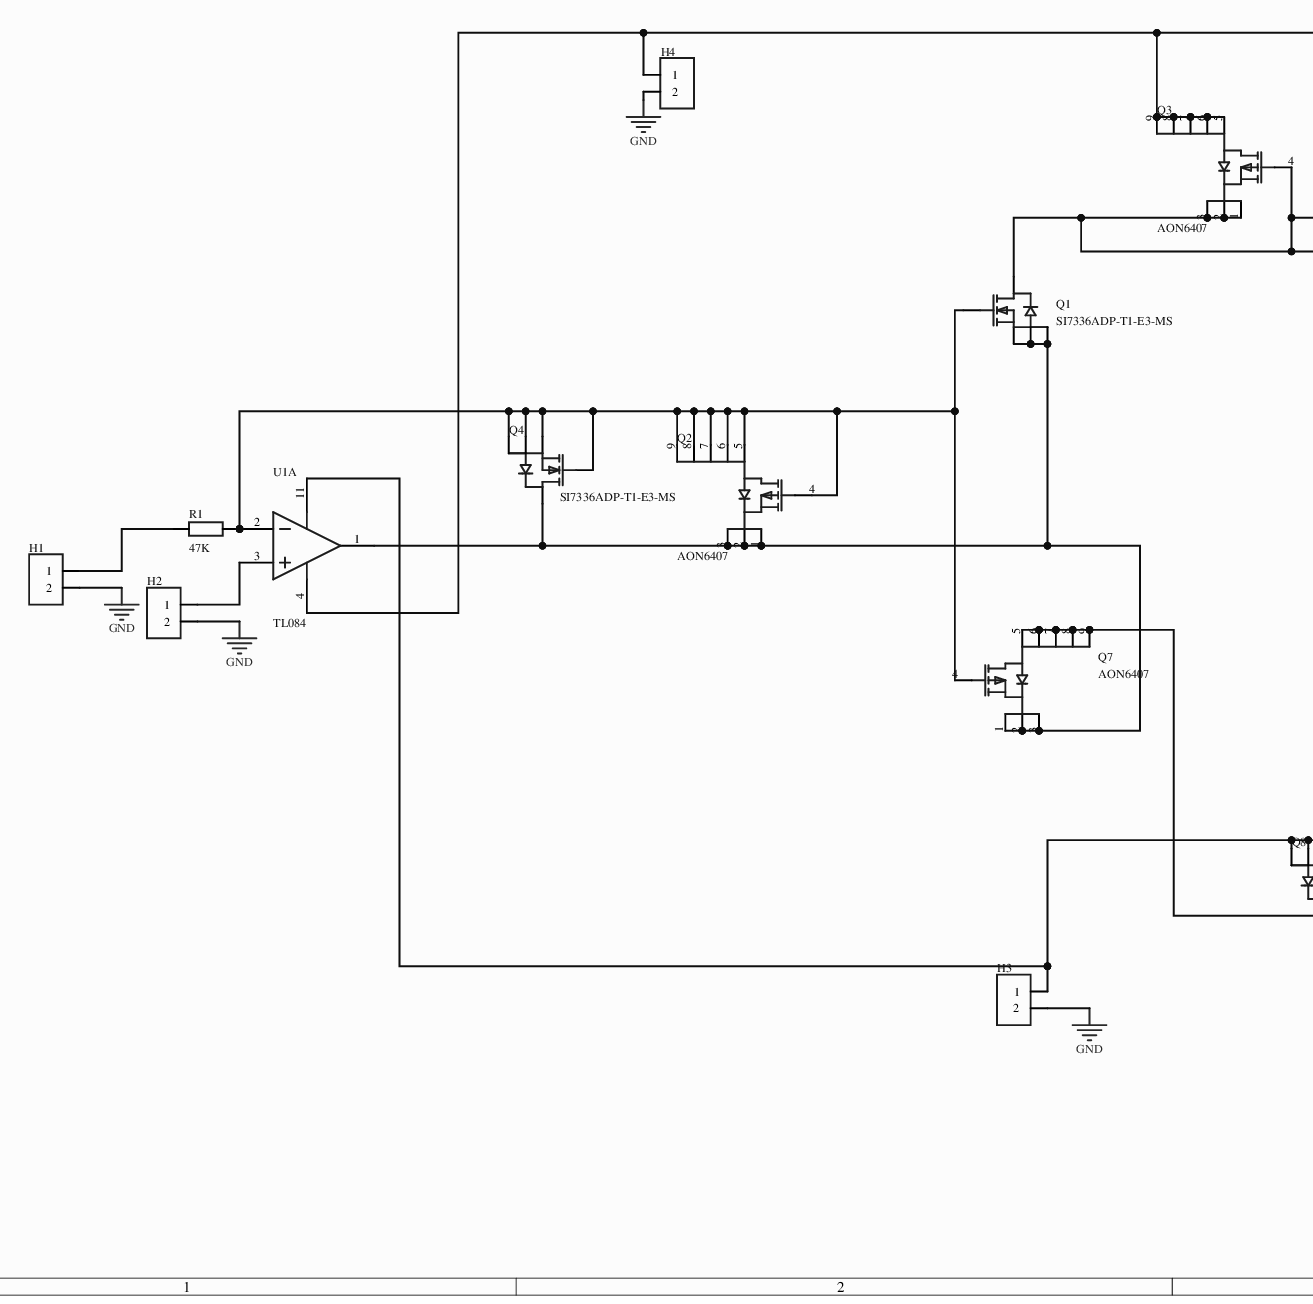
[diagram p0: MISC51994-3.schdoc, left]
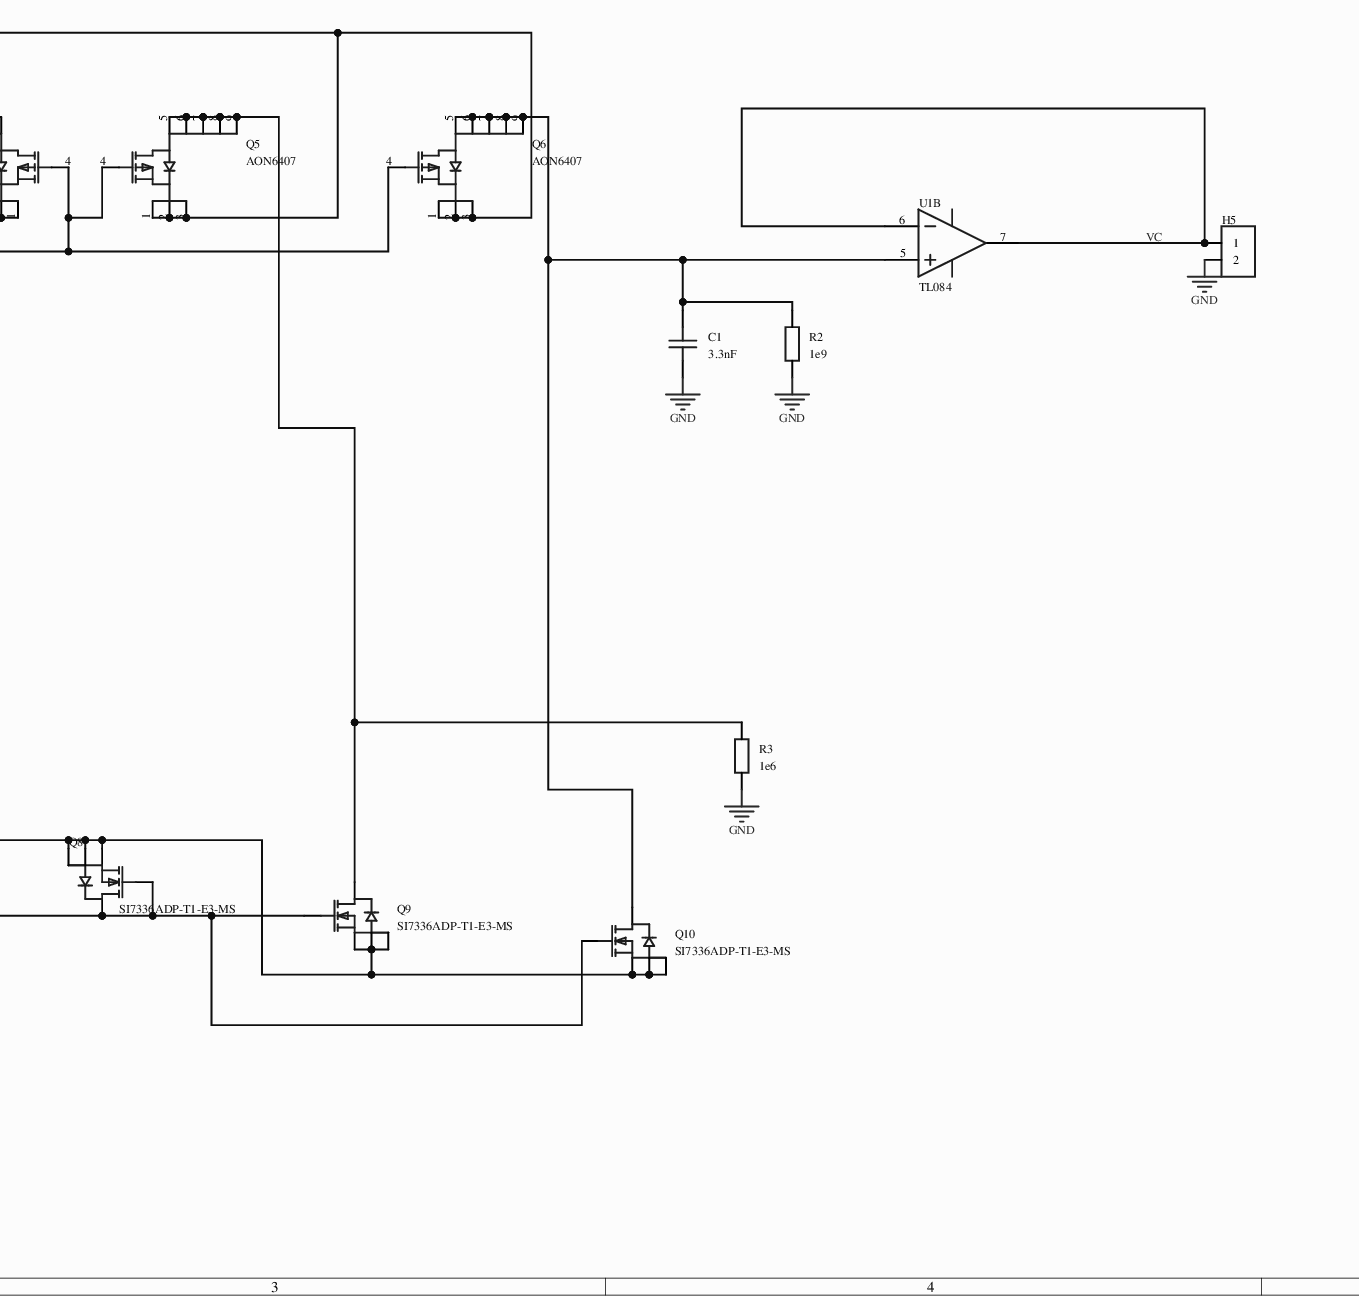
[diagram p1: MISC51994-3.schdoc, middle]
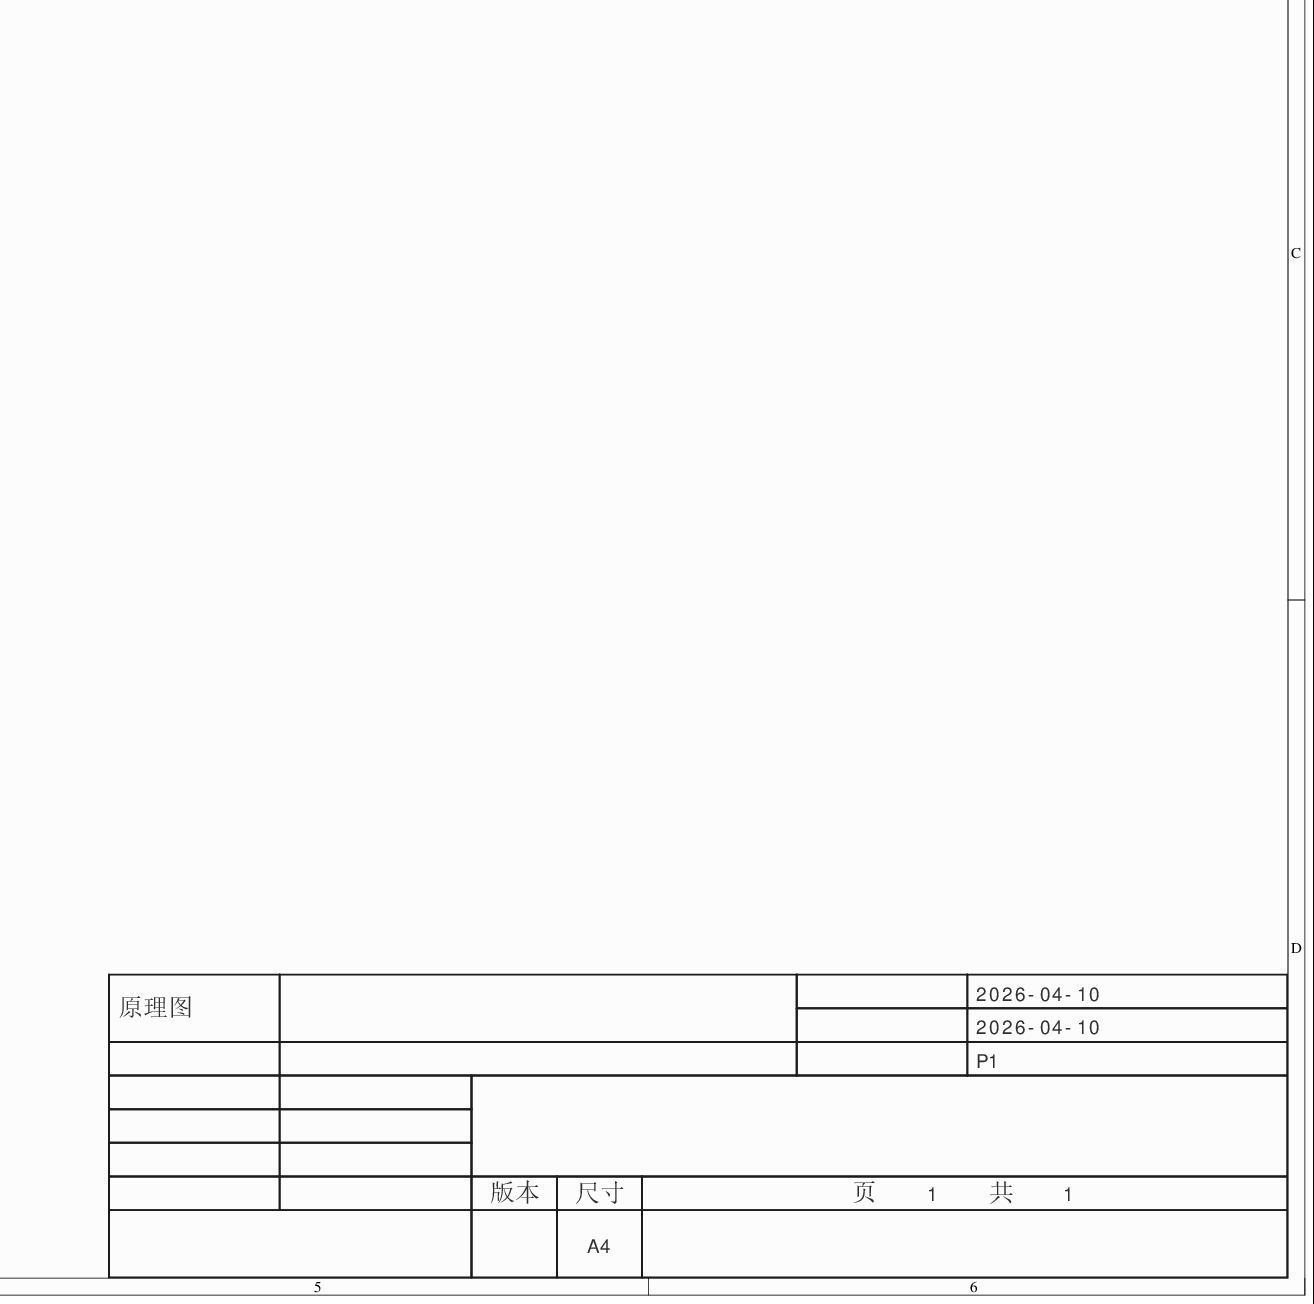
[diagram p2: MISC51994-3.schdoc, right]
# Altium project MISC51994-2.PrjPcb
1 sheet, 20 parts. Net scope: global (net labels, ports and power ports of the same name join across sheets).
Board file: MISC51994.pcbdoc

## Sheet MISC51994-3.schdoc
size 594 x 419 mm; Version: V1.0; @Project Name: MISC51994; @Update Date: 2026-04-10; @Create Date: 2026-04-10; @Board Name: MISC51994; @Create Time: 15:47:43; @Page Count: 1; @Page No: 1; @Schematic Name: MISC51994; @Update Time: 15:47:43; Size: A4

### Parts
C1  3.3nF  [C0805]
H1  (no value)  [HDR-TH_2P-P2.54-V-F]
H2  (no value)  [HDR-TH_2P-P2.54-V-F]
H3  (no value)  [HDR-TH_2P-P2.54-V-F]
H4  (no value)  [HDR-TH_2P-P2.54-V-F]
H5  (no value)  [HDR-TH_2P-P2.54-V-F]
Q1  SI7336ADP-T1-E3-MS  [TDSON-8_L5.9-W5.2-P1.27-BL-1]
Q2  AON6407  [PDFN-8_L4.9-W5.8-P1.27-LS6.1-BL]
Q3  AON6407  [PDFN-8_L4.9-W5.8-P1.27-LS6.1-BL]
Q4  SI7336ADP-T1-E3-MS  [TDSON-8_L5.9-W5.2-P1.27-BL-1]
Q5  AON6407  [PDFN-8_L4.9-W5.8-P1.27-LS6.1-BL]
Q6  AON6407  [PDFN-8_L4.9-W5.8-P1.27-LS6.1-BL]
Q7  AON6407  [PDFN-8_L4.9-W5.8-P1.27-LS6.1-BL]
Q8  SI7336ADP-T1-E3-MS  [TDSON-8_L5.9-W5.2-P1.27-BL-1]
Q9  SI7336ADP-T1-E3-MS  [TDSON-8_L5.9-W5.2-P1.27-BL-1]
Q10  SI7336ADP-T1-E3-MS  [TDSON-8_L5.9-W5.2-P1.27-BL-1]
R1  47K  [R0805]
R2  1e9  [R0805]
R3  1e6  [R0805]
U1  TL084  [SOP-14_L8.6-W3.9-P1.27-LS6.0-BL]  (parts A,B of 4)

### Nets
GND: C1.1 H1.2 H2.2 H3.2 H4.2 H5.2 R2.1 R3.1
VC: H5.1 U1.6(IN2-) U1.7(OUT2)
NetC1_2: C1.2 Q6.5(D) Q6.6(D) Q6.7(D) Q6.8(D) Q6.9(D) Q10.5(D) R2.2 U1.5(IN2+)
NetH1_1: H1.1 R1.1
NetH2_1: H2.1 U1.3(IN1+)
NetH3_1: H3.1 Q8.1(S) Q8.2(S) Q8.3(S) Q9.1(S) Q9.2(S) Q9.3(S) Q10.1(S) Q10.2(S) Q10.3(S) U1.11(VCC+)
NetH4_1: H4.1 Q3.5(D) Q3.6(D) Q3.7(D) Q3.8(D) Q3.9(D) Q5.1(S) Q5.2(S) Q5.3(S) Q6.1(S) Q6.2(S) Q6.3(S) U1.4(VCC-)
NetQ1_1: Q1.1(S) Q1.2(S) Q1.3(S) Q2.1(S) Q2.2(S) Q2.3(S) Q4.5(D) Q7.1(S) Q7.2(S) Q7.3(S) U1.1(OUT1)
NetQ1_4: Q1.4(G) Q2.4(G) Q2.5(D) Q2.6(D) Q2.7(D) Q2.8(D) Q2.9(D) Q4.1(S) Q4.2(S) Q4.3(S) Q4.4(G) Q7.4(G) R1.2 U1.2(IN1-)
NetQ1_5: Q1.5(D) Q3.1(S) Q3.2(S) Q3.3(S) Q3.4(G) Q5.4(G) Q6.4(G)
NetQ5_5: Q5.5(D) Q5.6(D) Q5.7(D) Q5.8(D) Q5.9(D) Q9.5(D) R3.2
NetQ7_5: Q7.5(D) Q7.6(D) Q7.7(D) Q7.8(D) Q7.9(D) Q8.4(G) Q8.5(D) Q9.4(G) Q10.4(G)

### Notes on the sheet
- 2026-04-10
- 原理图
- P1
- 版本
- 尺寸
- A4
- 页    1    共    1

### Library data of the parts
C1 = CAP_0805: Symbol: Capacitance; ConvertToPcb: yes; ModelId: 1ba041120af144c991958decab20d2410819f05c4eef4c71ace90d822a990e87; ModelName: C0805_L2.0-W1.3-H1.3; ModelTransform: 78.74,51.181,0,0,0,0,0,0.0005,0; Device: CAP_0805; Value: 3.3nF; AddInBom: yes; Supplier Footprint: 0805; FootprintName: C0805
H1-H5 = HDR-F_2.54_1x2P: Symbol: Header-Female-2.54_1x2; ConvertToPcb: yes; ModelId: a9450ef445564560a104363b9aacde4e0819f05c4eef4c71ace90d822a990e87; ModelName: HDR-TH_2P-P2.54-F-LI-1X2P; ModelTransform: 215.7476,98.425,0,0,0,0,0,0,-129.921; Device: HDR-F_2.54_1x2P; AddInBom: yes; SupplierPart: C49661; Supplier Footprint: 插件; FootprintName: HDR-TH_2P-P2.54-V-F
Q1 Q4 Q8-Q10 = SI7336ADP-T1-E3-MS: 此款SI7336ADP-T1-E3-MS是一款N沟道MOS管，采用紧凑型DFN5X6-8L封装，专为现代高集成度电子产品设计。器件在30V的最大漏源电压(VDSS)下运行，可承载高达150A的连续漏极电流(ID)，彰显其卓越的电力处理性能。导通电阻(RD(on))低至2mΩ，显著减少功率损耗，提升电路效率，广泛应用于电源转换、电机驱动等高功率场景，是您实现高效节能电路的理想半导体元件选择。; Manufacturer: MSKSEMI(美森科); AddInBom: yes; ModelId: 6d3ef2b64d5a4f2dbd2ee02e0c7053d20819f05c4eef4c71ace90d822a990e87; ModelTransform: 205.511,242.1255,0,0,0,0,0,42.913,0; Symbol: SI7336ADP-T1-E3-MS; Device: SI7336ADP-T1-E3-MS; LCSC Part Name: SI7336ADP-T1-E3-MS; SupplierPart: C51928007; ManufacturerPart: SI7336ADP-T1-E3-MS; Supplier Footprint: DFN-8L(5x6); JLCPCB Part Class: Extended Part; Datasheet: https://item.szlcsc.com/datasheet/SI7336ADP-T1-E3-MS/54639598.html; Supplier: LCSC; ConvertToPcb: yes; FootprintName: TDSON-8_L5.9-W5.2-P1.27-BL-1; ModelName: TDSON-8_L5.9-W5.2-P1.27-BL-1
Q2 Q3 Q5-Q7 = AON6407: 类型:1个P沟道;漏源电压(Vdss):30V;连续漏极电流(Id):85A;导通电阻(RDS(on)@Vgs,Id):4.5mΩ@10V,20A;功率(Pd):83W;阈值电压(Vgs(th)@Id):2.1V@250uA;; Manufacturer: AOS; AddInBom: yes; ModelId: 178189b27e7544aca50c1114265553580819f05c4eef4c71ace90d822a990e87; ModelName: PDFN-8_L4.9-W5.8-H1.0-P1.27; ModelTransform: 200.787,240.157,0,0,0,0,-0.097,0,0; Type: 1个P沟道; Drain Source Voltage (Vdss): 30V; Continuous Drain Current (Id): 85A; Power Dissipation (Pd): 83W; Total Gate Charge (Qg@Vgs): 105nC@10V; Input Capacitance (Ciss@Vds): 3.505nF@15V; Reverse Transfer Capacitance (Crss@Vds): 650pF@15V; Symbol: AON6407; Device: AON6407; LCSC Part Name: 1个P沟道 耐压:30V 电流:85A; SupplierPart: C13899; ManufacturerPart: AON6407; Supplier Footprint: PDFN-8(5.8x4.9); JLCPCB Part Class: Extended Part; Datasheet: https://atta.szlcsc.com/upload/public/pdf/source/20130618/1457706611203.pdf; Supplier: LCSC; ConvertToPcb: yes; FootprintName: PDFN-8_L4.9-W5.8-P1.27-LS6.1-BL; Drain Source On Resistance (RDS(on)@Vgs,Id): 4.5mΩ@10V,20A; Gate Threshold Voltage (Vgs(th)@Id): 2.1V@250uA; Operating Temperature: -55℃~+150℃
R1-R3 = Res_0805: Symbol: 电阻; ConvertToPcb: yes; ModelId: 37a81e68749a4138bd2dfa6897b24b850819f05c4eef4c71ace90d822a990e87; ModelName: R0805_L2.0-W1.3-H0.6; ModelTransform: 78.74,51.181,0,0,0,0,0,-0.0005,0; Device: Res_0805; AddInBom: yes; Supplier Footprint: 0805; FootprintName: R0805
  R1: Value: 47K
  R2: Value: 1e9
  R3: Value: 1e6
U1 = TL084: 放大器数:4;轨到轨:-;增益带宽积(GBW):-;输入失调电压(Vos):13mV;压摆率(SR):16V/us;输入偏置电流(Ib):20nA;; Manufacturer: Gcore(扬州国芯); Relevance: []; AddInBom: yes; ModelId: 520b569c4a2341089bdfdd9bf52b86190819f05c4eef4c71ace90d822a990e87; ModelTransform: 339.763,236.22,0,0,0,0,0,0,0; Number of Channels: 4; Maximum Power Supply Range (Vdd-Vss): 36V; Vos - Input Offset Voltage: 13mV; Slew Rate: 16V/us; Ib - Input Bias Current: 20nA; Input Offset Current(Ios): 4nA; Common Mode Rejection Ratio(CMRR): 75dB; Quiescent Current: 1.4mA; Output Current: 50mA; Dual Supply: -18V~18V; Symbol: TL084; Device: TL084; LCSC Part Name: TL084; SupplierPart: C504548; ManufacturerPart: TL084; Supplier Footprint: SOP-14; JLCPCB Part Class: Extended Part; Datasheet: https://item.szlcsc.com/datasheet/TL084/517189.html; Supplier: LCSC; ConvertToPcb: yes; FootprintName: SOP-14_L8.6-W3.9-P1.27-LS6.0-BL; ModelName: SOP-14_L8.6-W3.9-P1.27-LS6.0-BL; Rail to Rail: -; Gain Bandwidth Product: -; Input Offset Voltage Drift(Vos TC): -; Input Voltage Noise Density: -; Input offset current drift(Ios TC): -; Operating Temperature: 0℃~+70℃; Single supply: -; Features: -